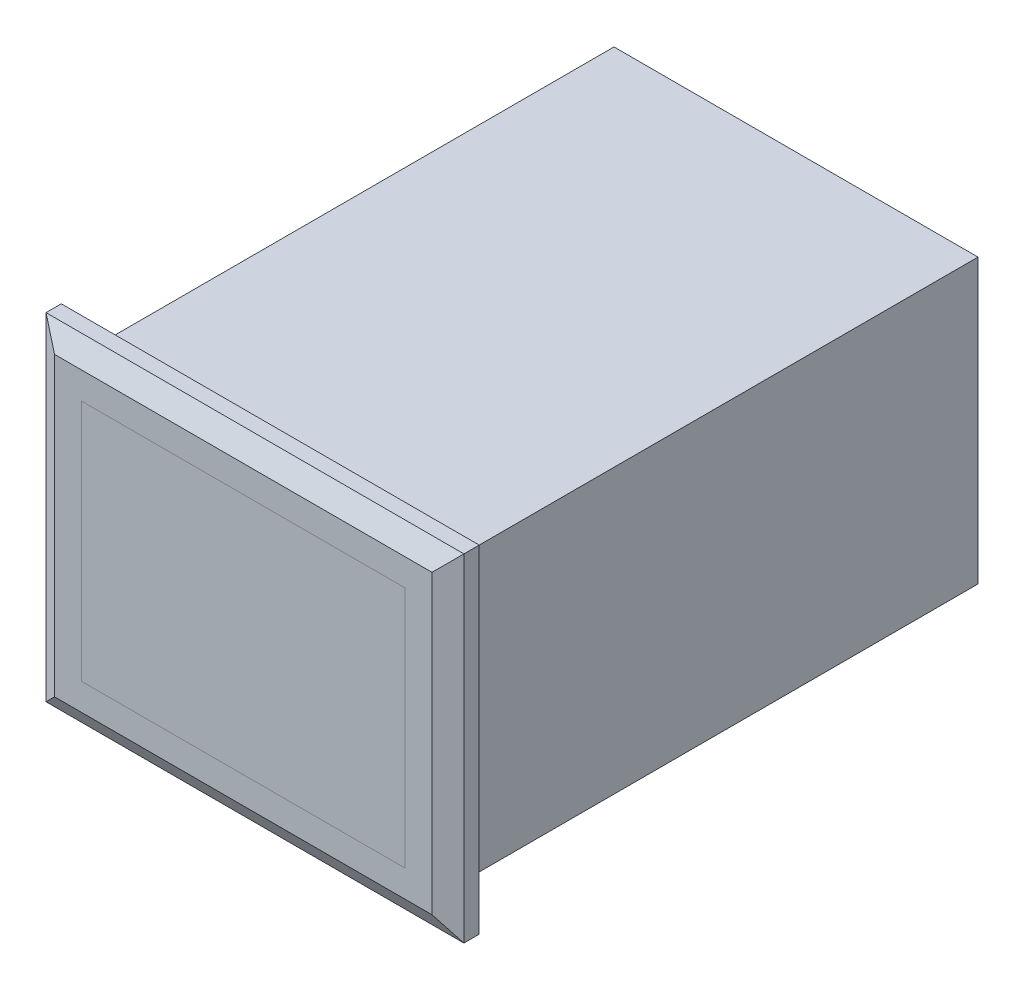
SolidWorks part; units mm, degrees
ref_plane "Front Plane" through (0, 0, 0) normal (0, 0, 1) x (1, 0, 0)
ref_plane "Top Plane" through (0, 0, 0) normal (0, 1, 0) x (1, 0, 0)
ref_plane "Right Plane" through (0, 0, 0) normal (1, 0, 0) x (0, 0, -1)
sketch "Sketch1" plane through (0, 0, 0) normal (0, 0, 1) x (1, 0, 0)
  line L1 (-13.5, -10.5) -> (13.5, -10.5)
  line L2 (-13.5, -10.5) -> (-13.5, 10.5)
  line L3 (-13.5, 10.5) -> (13.5, 10.5)
  line L4 (13.5, -10.5) -> (13.5, 10.5)
  line L5 (-13.5, -10.5) -> (13.5, 10.5) construction
  line L6 (-13.5, 10.5) -> (13.5, -10.5) construction
  point P0 (0, 0)
  dimension "D1" = 27
  dimension "D2" = 21
extrude "Boss-Extrude1" add sketch "Sketch1" along normal blind 39
sketch "Sketch2" plane through (0, 0, 39) normal (0, 0, 1) x (1, 0, 0)
  line L1 (-15.5, -12.5) -> (15.5, -12.5)
  line L2 (-15.5, -12.5) -> (-15.5, 12.5)
  line L3 (-15.5, 12.5) -> (15.5, 12.5)
  line L4 (15.5, -12.5) -> (15.5, 12.5)
  line L5 (-15.5, -12.5) -> (15.5, 12.5) construction
  line L6 (-15.5, 12.5) -> (15.5, -12.5) construction
  point P0 (0, 0)
  dimension "D1" = 31
  dimension "D2" = 25
extrude "Boss-Extrude2" add sketch "Sketch2" along normal blind 2
sketch "Sketch3" plane through (0, 0, 41) normal (0, 0, 1) x (1, 0, 0)
  line L1 (-12, -9) -> (12, -9)
  line L2 (-12, -9) -> (-12, 9)
  line L3 (-12, 9) -> (12, 9)
  line L4 (12, -9) -> (12, 9)
  line L5 (-12, -9) -> (12, 9) construction
  line L6 (-12, 9) -> (12, -9) construction
  point P0 (0, 0)
  dimension "D1" = 24
  dimension "D2" = 18
split line "Split Line1"
chamfer "Chamfer1" distance 1.5 angle 30 4 edges at (0, -12.5, 41) (-15.5, 0, 41) (15.5, 0, 41) (0, 12.5, 41)
